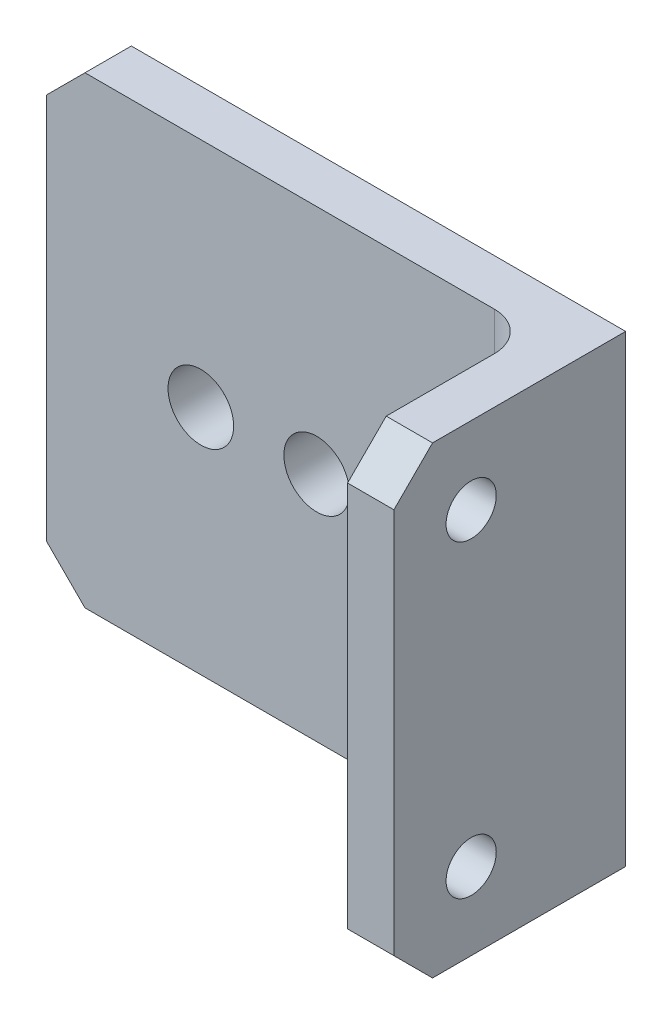
SolidWorks part; units mm, degrees
ref_plane "Front Plane" through (0, 0, 0) normal (0, 0, 1) x (1, 0, 0)
ref_plane "Top Plane" through (0, 0, 0) normal (0, 1, 0) x (1, 0, 0)
ref_plane "Right Plane" through (0, 0, 0) normal (1, 0, 0) x (0, 0, -1)
sketch "Sketch1" plane through (0, 0, 0) normal (0, 0, 1) x (1, 0, 0)
  line L1 (34.5, -30) -> (-34.5, -30)
  line L2 (34.5, -30) -> (34.5, 30)
  line L3 (34.5, 30) -> (-34.5, 30)
  line L4 (-34.5, -30) -> (-34.5, 30)
  line L5 (34.5, -30) -> (-34.5, 30) construction
  line L6 (34.5, 30) -> (-34.5, -30) construction
  point P0 (0, 0)
  dimension "D1" = 60
  dimension "D2" = 69
extrude "Boss-Extrude1" add sketch "Sketch1" along normal mid plane 6
sketch "Sketch2" plane through (0, 0, 3) normal (0, 0, 1) x (1, 0, 0)
  line L0 (-34.5, -30) -> (34.5, -30) construction
  line L1 (34.5, 30) -> (28.5, 30)
  line L2 (34.5, 30) -> (34.5, -30)
  line L3 (34.5, -30) -> (28.5, -30)
  line L4 (28.5, 30) -> (28.5, -30)
  dimension "D1" = 6
extrude "Boss-Extrude2" add sketch "Sketch2" along normal blind 24
chamfer "Chamfer1" distance 5 angle 45 4 edges at (-34.5, 30, 0) (-34.5, -30, 0) (31.5, 30, 27) (31.5, -30, 27)
sketch "Sketch3" plane through (0, 0, 3) normal (0, 0, 1) x (1, 0, 0)
  line L0 (-34.5, 0) -> (34.5, 0) construction
  line L1 (-34.5, 25) -> (-34.5, -25) construction
  line L2 (34.5, -25) -> (34.5, 25) construction
  circle A0 centre (-14.5, 0) radius 4.25
  circle A1 centre (0.5, 0) radius 4.25
  dimension "D1" = 20
  dimension "D2" = 15
  dimension "D3" = 8.5
extrude "Cut-Extrude1" cut sketch "Sketch3" against normal through all
fillet "Fillet1" radius 5 1 edges at (28.5, 0, 3)
sketch "Sketch4" plane through (28.5, 0, 0) normal (-1, 0, 0) x (0, 0, 1)
  line L0 (27, 25) -> (27, -25) construction
  line L1 (22, 30) -> (8, 30) construction
  circle A0 centre (17, 20) radius 3.25
  circle A1 centre (17, -20) radius 3.25
  dimension "D1" = 6.5
  dimension "D4" = 40
  dimension "D2" = 10
  dimension "D3" = 10
extrude "Cut-Extrude2" cut sketch "Sketch4" against normal through all
